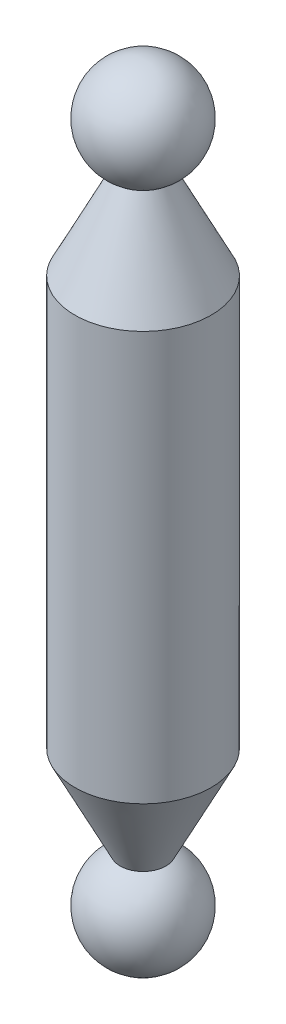
from build123d import *


with BuildPart() as part:
    # Sketch1 → Revolve1 (revolve)
    with BuildSketch(Plane.XY, mode=Mode.PRIVATE) as revolve1_sk:
        with BuildLine():
            Line((-3.354101966, 93.291796068), (-10, 80))
            Line((-10, 80), (-10, 20))
            Line((-10, 20), (-3.354101966, 6.708203932))
            ThreePointArc((-3.354101966, 6.708203932), (-7.299367421, -1.723146904), (0, -7.5))
            Line((0, -7.5), (0, 107.5))
            ThreePointArc((0, 107.5), (-7.299367421, 101.723146904), (-3.354101966, 93.291796068))
        make_face()
    revolve(revolve1_sk.sketch.rotate(Axis((0, -7.5, 0), (0, 1, 0)), 270), axis=Axis((0, -7.5, 0), (0, 1, 0)))


solid = part.part
